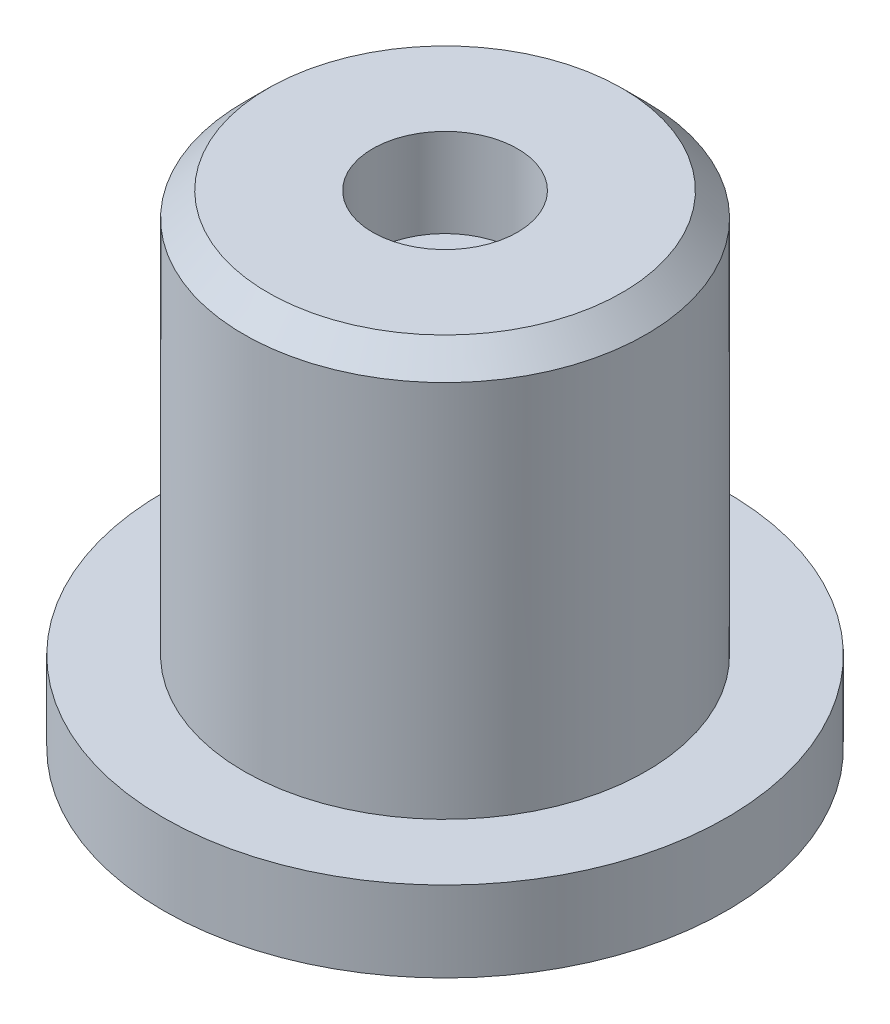
SolidWorks part; units mm, degrees
ref_plane "Front Plane" through (0, 0, 0) normal (0, 0, 1) x (1, 0, 0)
ref_plane "Top Plane" through (0, 0, 0) normal (0, 1, 0) x (1, 0, 0)
ref_plane "Right Plane" through (0, 0, 0) normal (1, 0, 0) x (0, 0, -1)
sketch "Sketch1" plane through (0, 0, 0) normal (0, 1, 0) x (1, 0, 0)
  circle A0 centre (0, 0) radius 35
  dimension "D1" = 70
extrude "Boss-Extrude1" add sketch "Sketch1" along normal blind 10
sketch "Sketch2" plane through (0, 10, 0) normal (0, 1, 0) x (1, 0, 0)
  circle A0 centre (0, 0) radius 25
  dimension "D1" = 50
extrude "Boss-Extrude2" add sketch "Sketch2" along normal blind 50
chamfer "Chamfer1" distance 3 angle 45 1 edges at (0, 60, 25)
sketch "Sketch3" plane through (0, 60, 0) normal (0, 1, 0) x (1, 0, 0)
  circle A0 centre (0, 0) radius 9
  dimension "D1" = 18
extrude "Cut-Extrude1" cut sketch "Sketch3" against normal blind 11
sketch "Sketch4" plane through (0, 49, 0) normal (0, 1, 0) x (1, 0, 0)
  circle A0 centre (0, 0) radius 5.5
  dimension "D1" = 11
extrude "Cut-Extrude2" cut sketch "Sketch4" against normal blind 76
